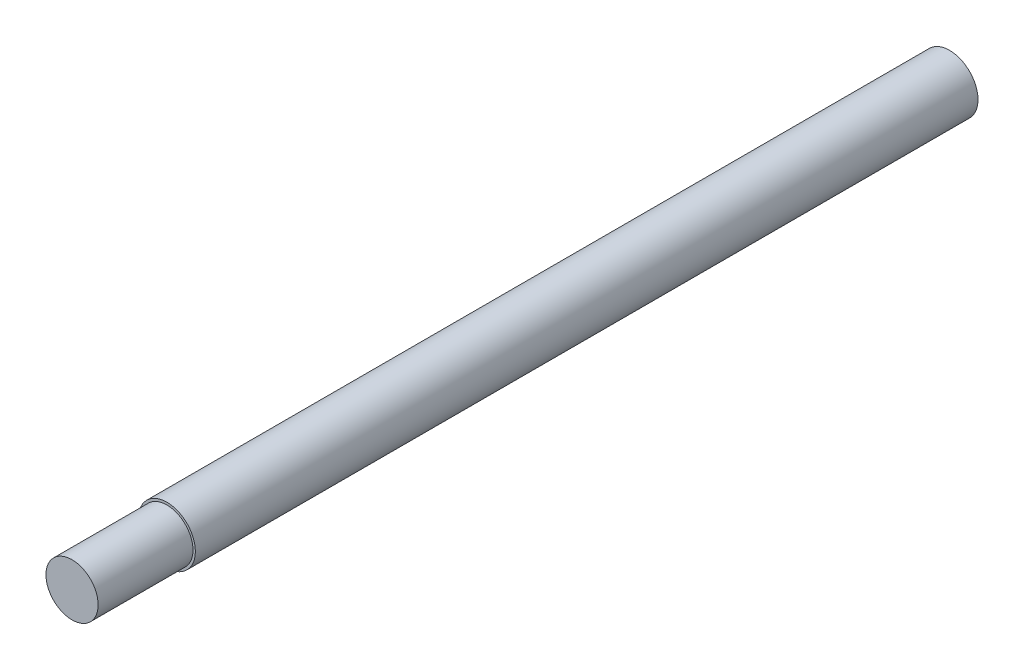
from build123d import *

# Parameters (mm, degrees)
SKETCH_1_R          = 6
EXTRUDE_3_DEPTH     = 92.5
SKETCH_3_R          = 6
SKETCH_3_R_2        = 5.5
CUT_EXTRUDE_1_DEPTH = 20


with BuildPart() as part:
    # 草图1 → 凸台-拉伸3 (new, symmetric)
    with BuildSketch(Plane.XY):
        Circle(SKETCH_1_R)
    extrude(amount=EXTRUDE_3_DEPTH, both=True)

    # 草图3 → 切除-拉伸1 (cut)
    with BuildSketch(Plane.XY.offset(92.5)):
        Circle(SKETCH_3_R)
        Circle(SKETCH_3_R_2, mode=Mode.SUBTRACT)
    extrude(amount=-CUT_EXTRUDE_1_DEPTH, mode=Mode.SUBTRACT)


solid = part.part
